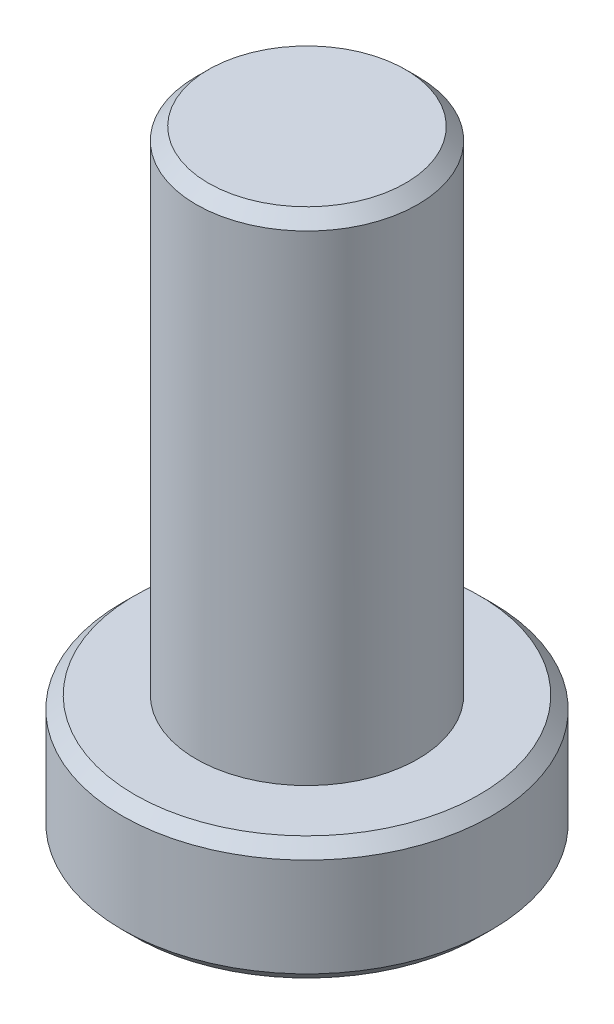
from build123d import *

# Parameters (mm, degrees)
CHAMFER1_SIZE = 0.5


with BuildPart() as part:
    # Sketch1 → Revolve1 (revolve)
    with BuildSketch(Plane(origin=(0, 0, 0), x_dir=(0, 0, -1), z_dir=(1, 0, 0))):
        Polygon((0, 25), (4.5, 25), (4.5, 5), (7.5, 5), (7.5, 0), (0, 0), align=None)
    revolve(axis=Axis((0, 0, 0), (0, 1, 0)))

    # Chamfer1
    chamfer1_edges = [part.edges().sort_by_distance(p)[0] for p in [
        (0, 0, 7.5),
        (0, 5, 7.5),
        (0, 25, 4.5),
    ]]
    chamfer(chamfer1_edges, length=CHAMFER1_SIZE)


solid = part.part
